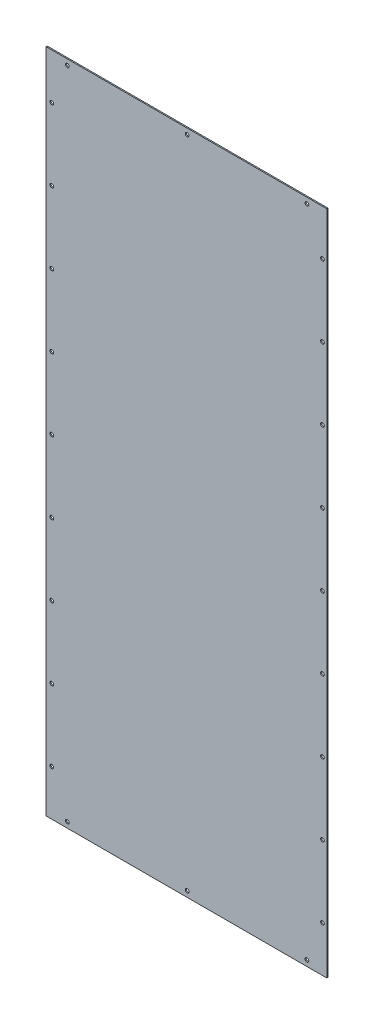
from build123d import *

# Parameters (mm, degrees)
SKETCH_1_W          = 494.5
SKETCH_1_H          = 1168
SKETCH_1_R          = 3.25
EXTRUDE_1_DEPTH     = 2
SKETCH_2_W          = 2.5
SKETCH_2_H          = 2
CUT_EXTRUDE_1_DEPTH = 1194.884652092


with BuildPart() as part:
    # 草图1 → 凸台-拉伸1 (new body)
    with BuildSketch(Plane.XY):
        Rectangle(SKETCH_1_W, SKETCH_1_H)
        with Locations((-237.25, 0)):
            Circle(SKETCH_1_R, mode=Mode.SUBTRACT)
        with Locations((-237.25, -126)):
            Circle(SKETCH_1_R, mode=Mode.SUBTRACT)
        with Locations((-237.25, -252)):
            Circle(SKETCH_1_R, mode=Mode.SUBTRACT)
        with Locations((-237.25, -378)):
            Circle(SKETCH_1_R, mode=Mode.SUBTRACT)
        with Locations((-237.25, -504)):
            Circle(SKETCH_1_R, mode=Mode.SUBTRACT)
        with Locations((0, -574)):
            Circle(SKETCH_1_R, mode=Mode.SUBTRACT)
        with Locations(Location((0, 574, 0), (0, 0, 180))):
            Circle(SKETCH_1_R, mode=Mode.SUBTRACT)
        with Locations(Location((-237.25, 504, 0), (0, 0, 180))):
            Circle(SKETCH_1_R, mode=Mode.SUBTRACT)
        with Locations(Location((-237.25, 378, 0), (0, 0, 180))):
            Circle(SKETCH_1_R, mode=Mode.SUBTRACT)
        with Locations(Location((-237.25, 252, 0), (0, 0, 180))):
            Circle(SKETCH_1_R, mode=Mode.SUBTRACT)
        with Locations(Location((-237.25, 126, 0), (0, 0, 180))):
            Circle(SKETCH_1_R, mode=Mode.SUBTRACT)
        with Locations((237.25, 126)):
            Circle(SKETCH_1_R, mode=Mode.SUBTRACT)
        with Locations((237.25, 252)):
            Circle(SKETCH_1_R, mode=Mode.SUBTRACT)
        with Locations((237.25, 378)):
            Circle(SKETCH_1_R, mode=Mode.SUBTRACT)
        with Locations((237.25, 504)):
            Circle(SKETCH_1_R, mode=Mode.SUBTRACT)
        with Locations(Location((237.25, -504, 0), (0, 0, 180))):
            Circle(SKETCH_1_R, mode=Mode.SUBTRACT)
        with Locations(Location((237.25, -378, 0), (0, 0, 180))):
            Circle(SKETCH_1_R, mode=Mode.SUBTRACT)
        with Locations(Location((237.25, -252, 0), (0, 0, 180))):
            Circle(SKETCH_1_R, mode=Mode.SUBTRACT)
        with Locations(Location((237.25, -126, 0), (0, 0, 180))):
            Circle(SKETCH_1_R, mode=Mode.SUBTRACT)
        with Locations(Location((237.25, 0, 0), (0, 0, 180))):
            Circle(SKETCH_1_R, mode=Mode.SUBTRACT)
        with Locations((-210, 574)):
            Circle(SKETCH_1_R, mode=Mode.SUBTRACT)
        with Locations((210, 574)):
            Circle(SKETCH_1_R, mode=Mode.SUBTRACT)
        with Locations(Location((-210, -574, 0), (0, 0, 180))):
            Circle(SKETCH_1_R, mode=Mode.SUBTRACT)
        with Locations(Location((210, -574, 0), (0, 0, 180))):
            Circle(SKETCH_1_R, mode=Mode.SUBTRACT)
    extrude(amount=EXTRUDE_1_DEPTH)

    # 草图2 → 切除-拉伸1 (cut, through all)
    with BuildSketch(Plane.XZ.offset(584)):
        with Locations((246, 1)):
            Rectangle(SKETCH_2_W, SKETCH_2_H)
    extrude(amount=-CUT_EXTRUDE_1_DEPTH, mode=Mode.SUBTRACT)


solid = part.part
